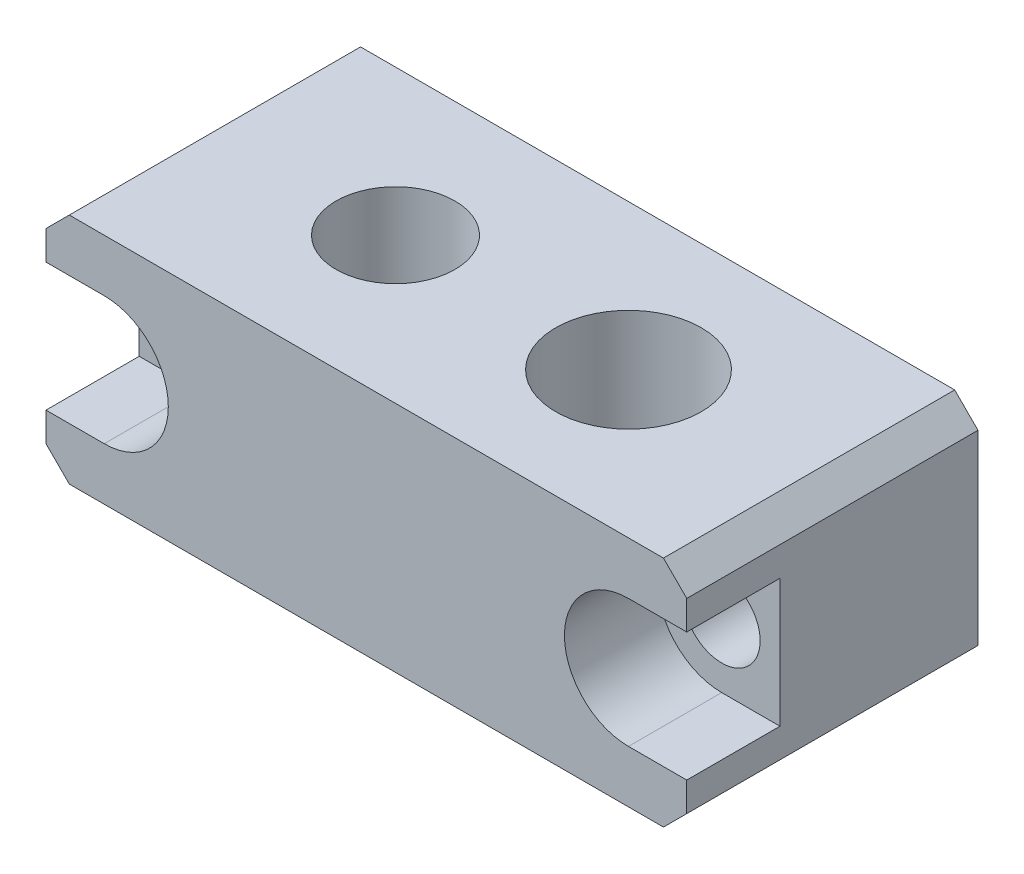
SolidWorks part; units mm, degrees
material "Q235-A"
ref_plane "Front Plane" through (0, 0, 0) normal (0, 0, 1) x (1, 0, 0)
ref_plane "Top Plane" through (0, 0, 0) normal (0, 1, 0) x (1, 0, 0)
ref_plane "Right Plane" through (0, 0, 0) normal (1, 0, 0) x (0, 0, -1)
sketch "Sketch1" plane through (0, 0, 0) normal (0, 0, 1) x (1, 0, 0)
  line L1 (-26.9507, 13.1105) -> (28.0493, 13.1105)
  line L2 (-26.9507, 13.1105) -> (-26.9507, -6.8895)
  line L3 (-26.9507, -6.8895) -> (28.0493, -6.8895)
  line L4 (28.0493, 13.1105) -> (28.0493, -6.8895)
  dimension "D1" = 55
  dimension "D2" = 20
extrude "Boss-Extrude1" add sketch "Sketch1" along normal blind 25
chamfer "Chamfer1" distance 2 angle 45 8 edges at (28.0493, 3.1105, 0) (28.0493, 3.1105, 25) (-26.9507, 3.1105, 0) (-26.9507, 3.1105, 25) (28.0493, 13.1105, 12.5) (28.0493, -6.8895, 12.5) (-26.9507, -6.8895, 12.5) (-26.9507, 13.1105, 12.5)
sketch "Sketch2" plane through (0, 0, 25) normal (0, 0, 1) x (1, 0, 0)
  line L0 (0.5493, 19.3929) -> (0.5493, -9.5845) construction
  line L1 (-26.9507, 3.1105) -> (28.0493, 3.1105) construction
  line L2 (-26.9507, 11.1105) -> (-26.9507, -4.8895) construction
  line L3 (28.0493, -4.8895) -> (28.0493, 11.1105) construction
  line L4 (-21.9507, 8.6105) -> (-26.9507, 8.6105)
  line L5 (-26.9507, 8.6105) -> (-26.9507, -2.3895)
  line L6 (-26.9507, -2.3895) -> (-21.9507, -2.3895)
  line L7 (23.0493, 8.6105) -> (28.0493, 8.6105)
  line L8 (28.0493, 8.6105) -> (28.0493, -2.3895)
  line L9 (28.0493, -2.3895) -> (23.0493, -2.3895)
  arc A0 (-21.9507, -2.3895) -> (-21.9507, 8.6105) centre (-21.9507, 3.1105) ccw
  arc A1 (23.0493, 8.6105) -> (23.0493, -2.3895) centre (23.0493, 3.1105) ccw
  dimension "D1" = 45
  dimension "D2" = 22.5
extrude "Cut-Extrude1" cut sketch "Sketch2" against normal blind 8
sketch "Sketch3" plane through (0, 0, 17) normal (0, 0, 1) x (1, 0, 0)
  line L0 (-21.9507, 3.1105) -> (23.0493, 3.1105)
hole_wizard "Hole1" positions "Sketch4" profile "Sketch5" legacy end condition through all
sketch "Sketch4" plane through (0, 0, 17) normal (0, 0, 1) x (1, 0, 0)
  point P0 (-21.9507, 3.1105)
  point P3 (23.0493, 3.1105)
sketch "Sketch5" plane through (-21.9507, 3.1105, 17) normal (1, 0, 0) x (0, -1, 0)
  line L0 (0, 0) -> (0, 17)
  line L1 (0, 17) -> (3.3, 17)
  line L2 (3.3, 17) -> (3.3, 0)
  line L3 (3.3, 0) -> (0, 0)
  line L4 (0, 110) -> (0, -10) construction
  dimension "直径" = 6.6
  dimension "深度" = 17
sketch "Sketch6" plane through (0, -6.8895, 0) normal (0, -1, 0) x (1, 0, 0)
  line L0 (-9.4507, 12.5) -> (10.5493, 12.5)
  line L1 (-24.9507, 0) -> (26.0493, 0) construction
  line L2 (-26.9507, 25) -> (-26.9507, 0) construction
  line L3 (28.0493, 25) -> (28.0493, 0) construction
  dimension "D1" = 12.5
  dimension "D2" = 17.5
  dimension "D3" = 17.5
hole_wizard "M12 Tapped Hole1" positions "Sketch7" profile "Sketch8" tap size "M12" standard "GB" end condition through all
sketch "Sketch7" plane through (0, -6.8895, 0) normal (0, -1, 0) x (-1, 0, 0)
  point P0 (9.4507, -12.5)
sketch "Sketch8" plane through (-9.4507, -6.8895, 12.5) normal (1, 0, 0) x (0, 0, -1)
  line L0 (0, 0) -> (0, 20)
  line L1 (0, 20) -> (5.1, 20)
  line L2 (5.1, 20) -> (5.1, 0)
  line L5 (5.1, 0) -> (0, 0)
  line L11 (0, -6.35) -> (0, 107.95) construction
  dimension "通孔螺纹孔钻头直径" = 10.2
  dimension "通孔螺纹孔钻头深度" = 20
cosmetic thread "Cosmetic thread 1" parameters "D2"=12
hole_wizard "M14x1.5 Tapped Hole1" positions "Sketch9" profile "Sketch10" tap size "M14x1.5" standard "GB" end condition through all
sketch "Sketch9" plane through (0, -6.8895, 0) normal (0, -1, 0) x (-1, 0, 0)
  point P0 (-10.5493, -12.5)
sketch "Sketch10" plane through (10.5493, -6.8895, 12.5) normal (1, 0, 0) x (0, 0, -1)
  line L0 (0, 0) -> (0, 20)
  line L1 (0, 20) -> (6.25, 20)
  line L2 (6.25, 20) -> (6.25, 0)
  line L5 (6.25, 0) -> (0, 0)
  line L11 (0, -6.35) -> (0, 107.95) construction
  dimension "通孔螺纹孔钻头直径" = 12.5
  dimension "通孔螺纹孔钻头深度" = 20
cosmetic thread "Cosmetic thread 2" parameters "D2"=14
